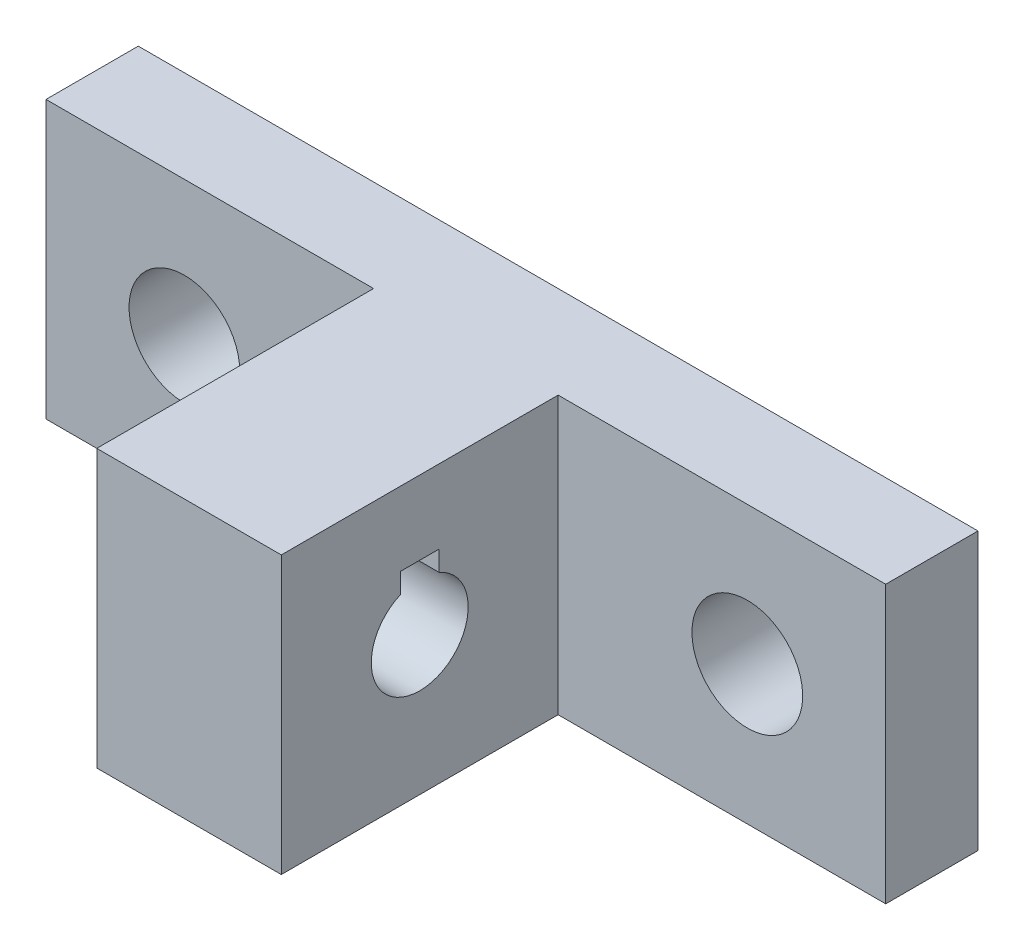
from build123d import *

# Parameters (mm, degrees)
SKETCH1_W           = 91
SKETCH1_H           = 30
BOSS_EXTRUDE1_DEPTH = 10
SKETCH2_W           = 20
SKETCH2_H           = 30
BOSS_EXTRUDE2_DEPTH = 30
CUT_EXTRUDE1_DEPTH  = 30
SKETCH5_R           = 6
CUT_EXTRUDE2_DEPTH  = 30


with BuildPart() as part:
    # Sketch1 → Boss-Extrude1 (new body)
    with BuildSketch(Plane.XY):
        Rectangle(SKETCH1_W, SKETCH1_H)
    extrude(amount=BOSS_EXTRUDE1_DEPTH)

    # Sketch2 → Boss-Extrude2 (add)
    with BuildSketch(Plane.XY.offset(10)):
        Rectangle(SKETCH2_W, SKETCH2_H)
    extrude(amount=BOSS_EXTRUDE2_DEPTH)

    # Sketch4 → Cut-Extrude1 (cut)
    with BuildSketch(Plane.ZY.offset(10)):
        with BuildLine():
            Line((27.1, 7), (22.9, 7))
            Line((22.9, 7), (22.9, 4.81170448))
            ThreePointArc((22.9, 4.81170448), (25, -5.25), (27.1, 4.81170448))
            Line((27.1, 4.81170448), (27.1, 7))
        make_face()
    extrude(amount=-CUT_EXTRUDE1_DEPTH, mode=Mode.SUBTRACT)

    # Sketch5 → Cut-Extrude2 (cut)
    with BuildSketch(Plane.XY.offset(10)):
        with Locations((-30.5, 0)):
            Circle(SKETCH5_R)
        with Locations(Location((30.5, 0, 0), (0, 0, 180))):
            Circle(SKETCH5_R)
    extrude(amount=-CUT_EXTRUDE2_DEPTH, mode=Mode.SUBTRACT)


solid = part.part
